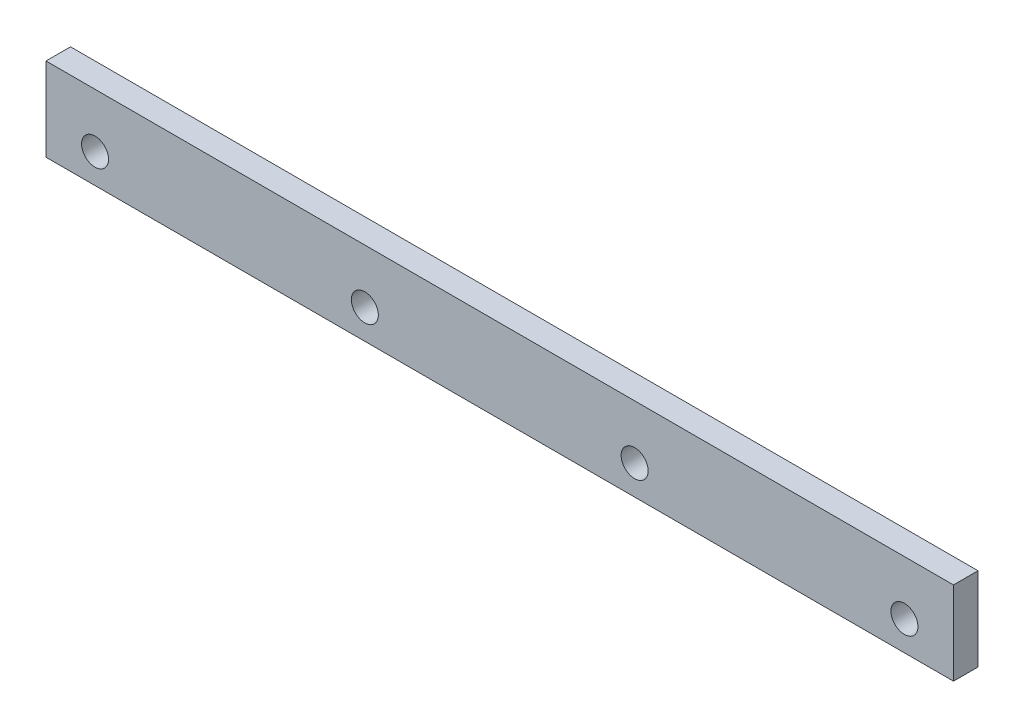
from build123d import *

# Parameters (mm, degrees)
SKETCH_1_W      = 370
SKETCH_1_H      = 34
SKETCH_1_R      = 5.5
EXTRUDE_1_DEPTH = 10


with BuildPart() as part:
    # 草图1 → 凸台-拉伸1 (new body)
    with BuildSketch(Plane.XY):
        Rectangle(SKETCH_1_W, SKETCH_1_H)
        with Locations((165, -5)):
            Circle(SKETCH_1_R, mode=Mode.SUBTRACT)
        with Locations((55, -5)):
            Circle(SKETCH_1_R, mode=Mode.SUBTRACT)
        with Locations((-55, -5)):
            Circle(SKETCH_1_R, mode=Mode.SUBTRACT)
        with Locations((-165, -5)):
            Circle(SKETCH_1_R, mode=Mode.SUBTRACT)
    extrude(amount=EXTRUDE_1_DEPTH)


solid = part.part
